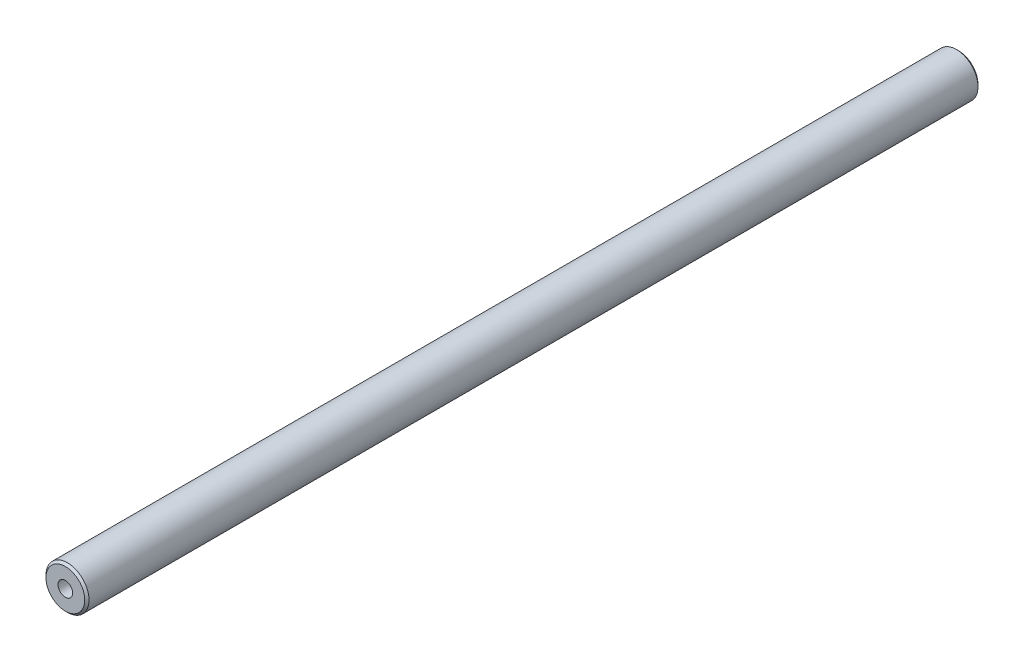
SolidWorks part; units mm, degrees
ref_plane "前视基准面" through (0, 0, 0) normal (0, 0, 1) x (1, 0, 0)
ref_plane "上视基准面" through (0, 0, 0) normal (0, 1, 0) x (1, 0, 0)
ref_plane "右视基准面" through (0, 0, 0) normal (1, 0, 0) x (0, 0, -1)
sketch "草图1" plane through (0, 0, 0) normal (0, 0, 1) x (1, 0, 0)
  circle A0 centre (0, 0) radius 10
  dimension "D1" = 20
extrude "凸台-拉伸1" add sketch "草图1" along normal blind 415
hole_wizard "M8 螺纹孔1" positions "草图3" profile "草图2" tap size "M8" standard "Gb"
sketch "草图3" plane through (0, 0, 415) normal (0, 0, 1) x (1, 0, 0)
  point P0 (0, 0)
sketch "草图2" plane through (0, 0, 415) normal (1, 0, 0) x (0, -1, 0)
  line L0 (0, 0) -> (0, 24.2929)
  line L1 (0, 24.2929) -> (3.4, 22.25)
  line L2 (3.4, 22.25) -> (3.4, 0)
  line L5 (3.4, 0) -> (0, 0)
  line L10 (0, 24.2929) -> (-3.4, 22.25) construction
  line L11 (0, -6.35) -> (0, 107.95) construction
  dimension "螺纹孔钻头直径" = 6.8
  dimension "螺纹孔钻头深度" = 22.25
  dimension "导头角度" = 118
cosmetic thread "孔螺蚊线1" parameters "D1"=16, "D2"=8
chamfer "倒角1" distance 1 angle 45 2 edges at (10, 0, 0) (10, 0, 415)
hole_wizard "M8 螺纹孔2" positions "草图5" profile "草图4" tap size "M8" standard "Gb"
sketch "草图5" plane through (0, 0, 0) normal (0, 0, -1) x (-1, 0, 0)
  point P0 (0, 0)
sketch "草图4" plane through (0, 0, 0) normal (1, 0, 0) x (0, 1, 0)
  line L0 (0, 0) -> (0, 24.2929)
  line L1 (0, 24.2929) -> (3.4, 22.25)
  line L2 (3.4, 22.25) -> (3.4, 0)
  line L5 (3.4, 0) -> (0, 0)
  line L10 (0, 24.2929) -> (-3.4, 22.25) construction
  line L11 (0, -6.35) -> (0, 107.95) construction
  dimension "螺纹孔钻头直径" = 6.8
  dimension "螺纹孔钻头深度" = 22.25
  dimension "导头角度" = 118
cosmetic thread "孔螺蚊线2" parameters "D1"=16, "D2"=8
